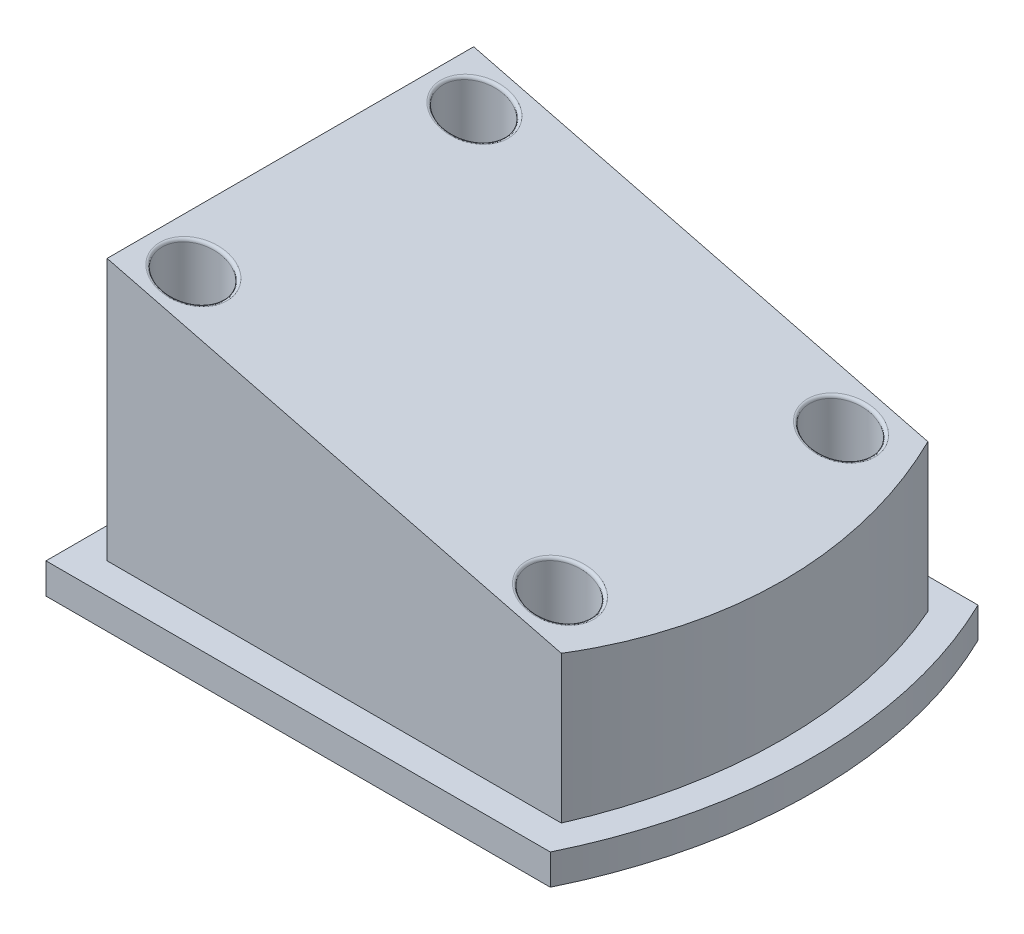
SolidWorks part; units mm, degrees
ref_plane "Front Plane" through (0, 0, 0) normal (0, 0, 1) x (1, 0, 0)
ref_plane "Top Plane" through (0, 0, 0) normal (0, 1, 0) x (1, 0, 0)
ref_plane "Right Plane" through (0, 0, 0) normal (1, 0, 0) x (0, 0, -1)
sketch "Sketch1" plane through (0, 0, 0) normal (0, 1, 0) x (1, 0, 0)
  line L1 (-41.27, 35) -> (41.27, 35)
  line L2 (-41.27, 35) -> (-41.27, -35)
  line L3 (-41.27, -35) -> (41.27, -35)
  line L4 (41.27, 35) -> (41.27, -35) construction
  line L5 (-41.27, 35) -> (41.27, -35) construction
  line L6 (-41.27, -35) -> (41.27, 35) construction
  arc A0 (41.27, 35) -> (41.27, -35) centre (-30.6675, 0) cw
  point P0 (0, 0)
  dimension "D1" = 70
  dimension "D3" = 80
  dimension "D2" = 82.54
extrude "Boss-Extrude1" add sketch "Sketch1" along normal blind 5
sketch "Sketch2" plane through (0, 5, 0) normal (0, 1, 0) x (1, 0, 0)
  line L3 (41.27, 35) -> (-41.27, 35)
  line L4 (-41.27, 35) -> (-41.27, -35)
  line L5 (-41.27, -35) -> (41.27, -35)
  line L6 (41.27, 35) -> (-41.27, 35) construction
  line L7 (-41.27, 35) -> (-41.27, -35) construction
  line L8 (-41.27, -35) -> (41.27, -35) construction
  line L12 (38.0712, 30) -> (-36.27, 30)
  line L13 (-36.27, 30) -> (-36.27, -30)
  line L14 (-36.27, -30) -> (38.0712, -30)
  line L15 (38.0712, 30) -> (-36.27, 30)
  line L16 (-36.27, 30) -> (-36.27, -30)
  line L17 (-36.27, -30) -> (38.0712, -30)
  arc A1 (41.27, -35) -> (41.27, 35) centre (-30.6675, 0) ccw
  arc A2 (41.27, -35) -> (41.27, 35) centre (-30.6675, 0) ccw construction
  arc A4 (38.0712, -30) -> (38.0712, 30) centre (-30.6675, 0) ccw
  arc A5 (38.0712, -30) -> (38.0712, 30) centre (-30.6675, 0) ccw
  dimension "D1" = 0
  dimension "D2" = 5
extrude "Boss-Extrude2" add sketch "Sketch2" along normal blind 42.87
sketch "Sketch3" plane through (0, 0, 30) normal (0, 0, 1) x (1, 0, 0)
  line L0 (44.3325, 5) -> (44.3325, 27.48)
  line L1 (44.3325, 5) -> (44.3325, 47.87) construction
  line L2 (-36.27, 5) -> (-36.27, 47.87)
  line L4 (-36.27, 47.87) -> (-36.27, 5) construction
  line L5 (-36.27, 47.87) -> (44.3325, 27.48)
  dimension "D1" = 22.48
  dimension "D2" = 42.87
extrude "Cut-Extrude1" cut sketch "Sketch3" against normal through all and the other way through all flip side to cut
sketch "Sketch5" plane through (0, 0, 0) normal (0, -1, 0) x (1, 0, 0)
  line L0 (-41.27, 35) -> (41.27, 35) construction
  line L1 (-41.27, -35) -> (-41.27, 35) construction
  line L2 (-1000, 0) -> (49000, 0) construction
  circle A0 centre (-29.27, 23) radius 5
  circle A1 centre (30.73, 23) radius 5
  circle A2 centre (30.73, -23) radius 5
  circle A3 centre (-29.27, -23) radius 5
  dimension "D1" = 10
  dimension "D2" = 12
  dimension "D3" = 12
  dimension "D4" = 60
extrude "Cut-Extrude2" cut sketch "Sketch5" against normal up to next from offset 20 contours A1 | A2 | A3 | A0 offset against normal yes
sketch "Sketch6" plane through (0, 5, 0) normal (0, 1, 0) x (1, 0, 0)
  circle A0 centre (-29.27, 23) radius 3
  circle A1 centre (30.73, 23) radius 3
  circle A2 centre (-29.27, -23) radius 3
  circle A3 centre (30.73, -23) radius 3
  dimension "D1" = 6
extrude "Cut-Extrude3" cut sketch "Sketch6" along normal up to next from offset 5
fillet "Fillet1" radius 0.5 4 edges at (35.73, 29.6562, 23) (35.73, 29.6562, -23) (-24.27, 44.8344, -23) (-24.27, 44.8344, 23)
